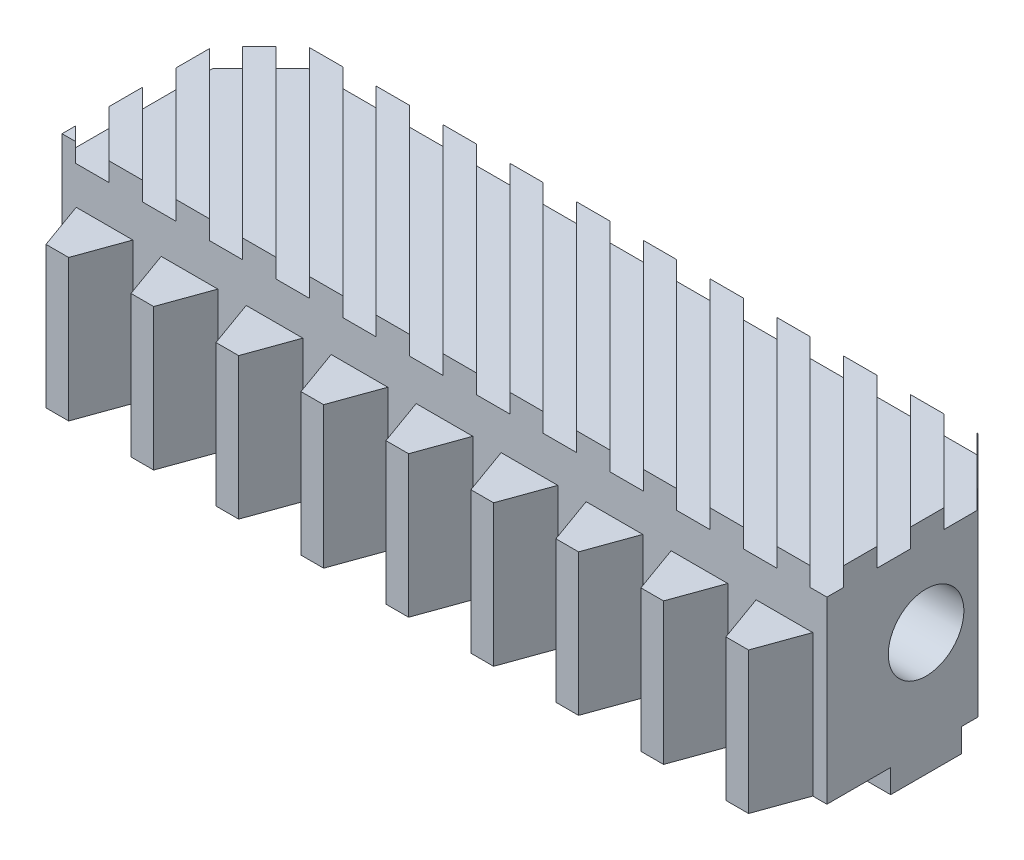
from build123d import *

# Parameters (mm, degrees)
BOSS_EXTRUDE1_DEPTH     = 30
SKETCH6_W               = 162
SKETCH6_H               = 42
BOSS_EXTRUDE2_DEPTH     = 12
CUT_EXTRUDE1_DEPTH      = 173.545646135
CUT_EXTRUDE1_DEPTH_BACK = 173.545646135
SKETCH7_R               = 8
SKETCH10_W              = 162
SKETCH10_H              = 15
BOSS_EXTRUDE3_DEPTH     = 5
CUT_EXTRUDE3_DEPTH      = 4
CHAMFER1_SIZE           = 10


with BuildPart() as part:
    # Sketch1 → Boss-Extrude1 (new body)
    with BuildSketch(Plane(origin=(0, 0, 0), x_dir=(1, 0, 0), z_dir=(0, 1, 0))):
        Polygon((0, 0), (3.6, -10), (8.4, -10), (12, 0), (18, 0), (21.6, -10), (26.4, -10), (30, 0), (36, 0), (39.6, -10), (44.4, -10), (48, 0), (54, 0), (57.6, -10), (62.4, -10), (66, 0), (72, 0), (75.6, -10), (80.4, -10), (84, 0), (90, 0), (93.6, -10), (98.4, -10), (102, 0), (108, 0), (111.6, -10), (116.4, -10), (120, 0), (126, 0), (129.6, -10), (134.4, -10), (138, 0), (144, 0), (147.6, -10), (152.4, -10), (156, 0), (159, 0), (159, 42), (-3, 42), (-3, 0), align=None)
    extrude(amount=BOSS_EXTRUDE1_DEPTH)

    # Sketch6 → Boss-Extrude2 (add)
    with BuildSketch(Plane(origin=(0, 30, 0), x_dir=(1, 0, 0), z_dir=(0, 1, 0))):
        with Locations((78, 21)):
            Rectangle(SKETCH6_W, SKETCH6_H)
    extrude(amount=BOSS_EXTRUDE2_DEPTH)

    # Sketch7 → Cut-Extrude1 (cut, two sides: drawn at the far end of the back side and taken through both)
    with BuildSketch(Plane.ZY.offset(3).offset(-CUT_EXTRUDE1_DEPTH_BACK)):
        with Locations((-21, 21)):
            Circle(SKETCH7_R)
    extrude(amount=CUT_EXTRUDE1_DEPTH + CUT_EXTRUDE1_DEPTH_BACK, mode=Mode.SUBTRACT)

    # Sketch10 → Boss-Extrude3 (add)
    with BuildSketch(Plane.XZ):
        with Locations((78, -21)):
            Rectangle(SKETCH10_W, SKETCH10_H)
    extrude(amount=BOSS_EXTRUDE3_DEPTH)

    # Sketch12 → Cut-Extrude3 (cut)
    with BuildSketch(Plane(origin=(0, 42, 0), x_dir=(1, 0, 0), z_dir=(0, 1, 0))):
        with BuildLine():
            Line((50.295857363, 112.239676543), (223.712429664, -61.176895758))
            ThreePointArc((223.712429664, -61.176895758), (223.712429664, -64.712429664), (220.176895758, -64.712429664))
            Line((220.176895758, -64.712429664), (46.760323457, 108.704142637))
            ThreePointArc((46.760323457, 108.704142637), (46.760323457, 112.239676543), (50.295857363, 112.239676543))
        make_face()
        with BuildLine():
            Line((53.831391269, 115.775210449), (227.24796357, -57.641361852))
            ThreePointArc((227.24796357, -57.641361852), (230.783497476, -57.641361852), (230.783497476, -54.105827946))
            Line((230.783497476, -54.105827946), (57.366925175, 119.310744355))
            ThreePointArc((57.366925175, 119.310744355), (53.831391269, 119.310744355), (53.831391269, 115.775210449))
        make_face()
        with BuildLine():
            Line((60.902459081, 122.846278261), (234.319031382, -50.57029404))
            ThreePointArc((234.319031382, -50.57029404), (237.854565288, -50.57029404), (237.854565288, -47.034760134))
            Line((237.854565288, -47.034760134), (64.437992987, 126.381812167))
            ThreePointArc((64.437992987, 126.381812167), (60.902459081, 126.381812167), (60.902459081, 122.846278261))
        make_face()
        with BuildLine():
            Line((67.973526893, 129.917346072), (241.390099194, -43.499226229))
            ThreePointArc((241.390099194, -43.499226229), (244.9256331, -43.499226229), (244.9256331, -39.963692323))
            Line((244.9256331, -39.963692323), (71.509060799, 133.452879978))
            ThreePointArc((71.509060799, 133.452879978), (67.973526893, 133.452879978), (67.973526893, 129.917346072))
        make_face()
        with BuildLine():
            Line((39.689255645, 101.633074825), (213.105827946, -71.783497476))
            ThreePointArc((213.105827946, -71.783497476), (216.641361852, -71.783497476), (216.641361852, -68.24796357))
            Line((216.641361852, -68.24796357), (43.224789551, 105.168608731))
            ThreePointArc((43.224789551, 105.168608731), (39.689255645, 105.168608731), (39.689255645, 101.633074825))
        make_face()
        with BuildLine():
            Line((32.618187833, 94.562007013), (206.034760134, -78.854565288))
            ThreePointArc((206.034760134, -78.854565288), (209.57029404, -78.854565288), (209.57029404, -75.319031382))
            Line((209.57029404, -75.319031382), (36.153721739, 98.097540919))
            ThreePointArc((36.153721739, 98.097540919), (32.618187833, 98.097540919), (32.618187833, 94.562007013))
        make_face()
        with BuildLine():
            Line((25.547120022, 87.490939201), (198.963692323, -85.9256331))
            ThreePointArc((198.963692323, -85.9256331), (202.499226229, -85.9256331), (202.499226229, -82.390099194))
            Line((202.499226229, -82.390099194), (29.082653928, 91.026473107))
            ThreePointArc((29.082653928, 91.026473107), (25.547120022, 91.026473107), (25.547120022, 87.490939201))
        make_face()
        with BuildLine():
            Line((18.47605221, 80.419871389), (191.892624511, -92.996700912))
            ThreePointArc((191.892624511, -92.996700912), (195.428158417, -92.996700912), (195.428158417, -89.461167006))
            Line((195.428158417, -89.461167006), (22.011586116, 83.955405295))
            ThreePointArc((22.011586116, 83.955405295), (18.47605221, 83.955405295), (18.47605221, 80.419871389))
        make_face()
        with BuildLine():
            Line((11.404984398, 73.348803578), (184.821556699, -100.067768723))
            ThreePointArc((184.821556699, -100.067768723), (188.357090605, -100.067768723), (188.357090605, -96.532234817))
            Line((188.357090605, -96.532234817), (14.940518304, 76.884337483))
            ThreePointArc((14.940518304, 76.884337483), (11.404984398, 76.884337483), (11.404984398, 73.348803578))
        make_face()
        with BuildLine():
            Line((4.333916586, 66.277735766), (177.750488887, -107.138836535))
            ThreePointArc((177.750488887, -107.138836535), (181.286022793, -107.138836535), (181.286022793, -103.603302629))
            Line((181.286022793, -103.603302629), (7.869450492, 69.813269672))
            ThreePointArc((7.869450492, 69.813269672), (4.333916586, 69.813269672), (4.333916586, 66.277735766))
        make_face()
        with BuildLine():
            Line((-2.737151226, 59.206667954), (170.679421075, -114.209904347))
            ThreePointArc((170.679421075, -114.209904347), (174.214954981, -114.209904347), (174.214954981, -110.674370441))
            Line((174.214954981, -110.674370441), (0.79838268, 62.74220186))
            ThreePointArc((0.79838268, 62.74220186), (-2.737151226, 62.74220186), (-2.737151226, 59.206667954))
        make_face()
        with BuildLine():
            Line((-9.808219038, 52.135600142), (163.608353263, -121.280972159))
            ThreePointArc((163.608353263, -121.280972159), (167.143887169, -121.280972159), (167.143887169, -117.745438253))
            Line((167.143887169, -117.745438253), (-6.272685132, 55.671134048))
            ThreePointArc((-6.272685132, 55.671134048), (-9.808219038, 55.671134048), (-9.808219038, 52.135600142))
        make_face()
        with BuildLine():
            Line((-16.87928685, 45.06453233), (156.537285451, -128.352039971))
            ThreePointArc((156.537285451, -128.352039971), (160.072819357, -128.352039971), (160.072819357, -124.816506065))
            Line((160.072819357, -124.816506065), (-13.343752944, 48.600066236))
            ThreePointArc((-13.343752944, 48.600066236), (-16.87928685, 48.600066236), (-16.87928685, 45.06453233))
        make_face()
        with BuildLine():
            Line((-23.950354661, 37.993464518), (149.46621764, -135.423107783))
            ThreePointArc((149.46621764, -135.423107783), (153.001751545, -135.423107783), (153.001751545, -131.887573877))
            Line((153.001751545, -131.887573877), (-20.414820756, 41.528998424))
            ThreePointArc((-20.414820756, 41.528998424), (-23.950354661, 41.528998424), (-23.950354661, 37.993464518))
        make_face()
        with BuildLine():
            Line((-31.021422473, 30.922396706), (142.395149828, -142.494175595))
            ThreePointArc((142.395149828, -142.494175595), (145.930683734, -142.494175595), (145.930683734, -138.958641689))
            Line((145.930683734, -138.958641689), (-27.485888567, 34.457930612))
            ThreePointArc((-27.485888567, 34.457930612), (-31.021422473, 34.457930612), (-31.021422473, 30.922396706))
        make_face()
        with BuildLine():
            Line((-38.092490285, 23.851328894), (135.324082016, -149.565243406))
            ThreePointArc((135.324082016, -149.565243406), (138.859615922, -149.565243406), (138.859615922, -146.029709501))
            Line((138.859615922, -146.029709501), (-34.556956379, 27.3868628))
            ThreePointArc((-34.556956379, 27.3868628), (-38.092490285, 27.3868628), (-38.092490285, 23.851328894))
        make_face()
    extrude(amount=-CUT_EXTRUDE3_DEPTH, mode=Mode.SUBTRACT)

    # Chamfer1
    chamfer1_edges = [part.edges().sort_by_distance(p)[0] for p in [
        (-3, 21, -42),
        (159, 19, -42),
    ]]
    chamfer(chamfer1_edges, length=CHAMFER1_SIZE)


solid = part.part
